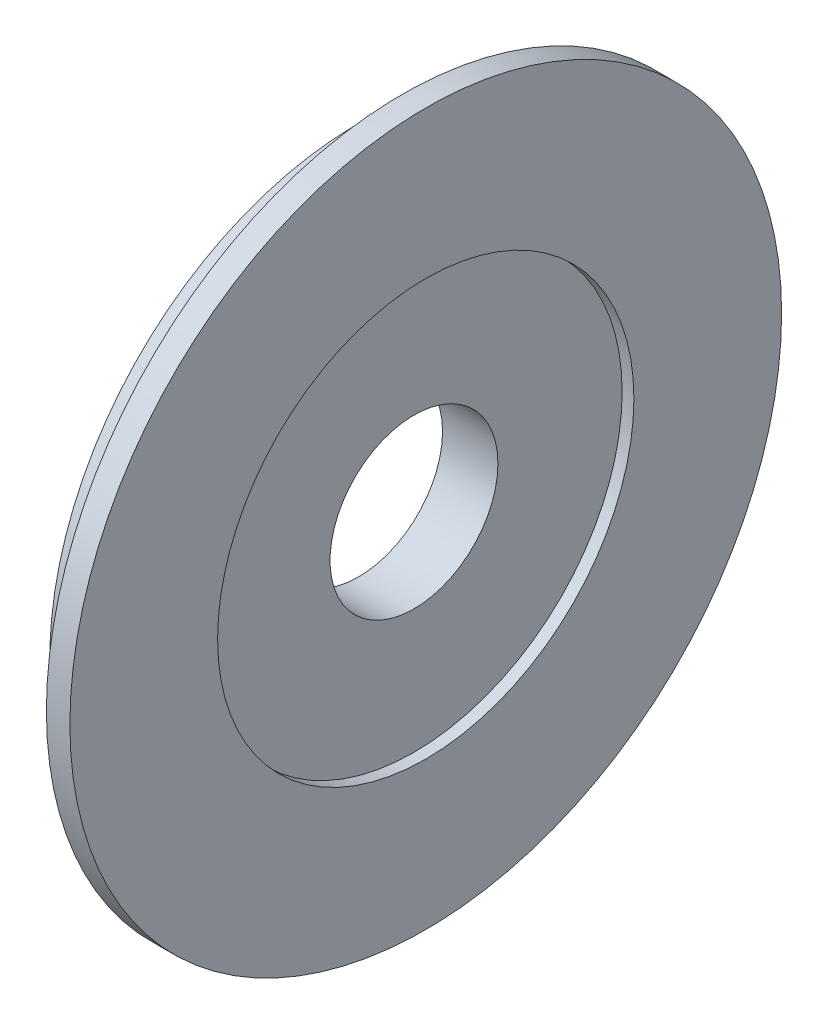
SolidWorks part; units mm, degrees
ref_plane "Front Plane" through (0, 0, 0) normal (0, 0, 1) x (1, 0, 0)
ref_plane "Top Plane" through (0, 0, 0) normal (0, 1, 0) x (1, 0, 0)
ref_plane "Right Plane" through (0, 0, 0) normal (1, 0, 0) x (0, 0, -1)
sketch "Sketch1" plane through (0, 0, 0) normal (0, 0, 1) x (1, 0, 0)
  line L0 (-11.7708, 46) -> (-11.7708, 12.5)
  line L7 (-3.5208, 31) -> (-1.7708, 31)
  line L8 (-1.7708, 31) -> (-1.7708, 53)
  line L9 (-1.7708, 53) -> (-5.2708, 53)
  line L10 (-5.2708, 53) -> (-7.7708, 46)
  line L11 (-7.7708, 46) -> (-11.7708, 46)
  line L12 (0, 0) -> (-40.9375, 0) construction
  line L13 (-11.7708, 12.5) -> (-3.5208, 12.5)
  line L14 (-3.5208, 12.5) -> (-3.5208, 31)
  dimension "D1" = 46
  dimension "D2" = 53
  dimension "D3" = 31
  dimension "D4" = 4
  dimension "D5" = 10
  dimension "D8" = 3.5
  dimension "D9" = 12.5
revolve "Revolve1" add sketch "Sketch1" angle 360 about L12
